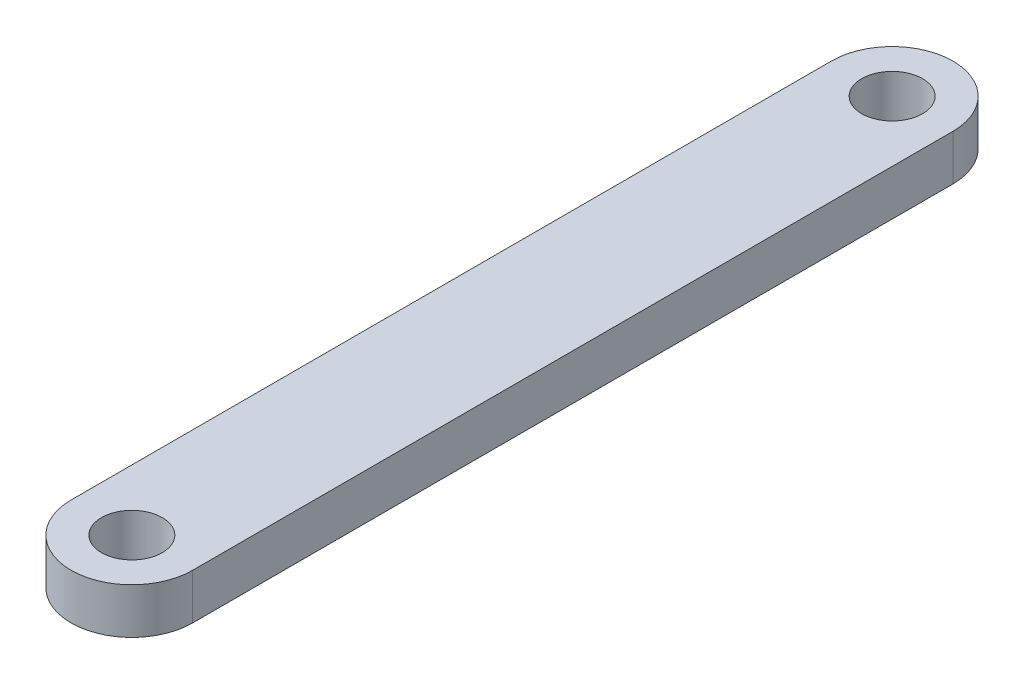
from build123d import *

# Parameters (mm, degrees)
SKETCH1_R           = 10
BOSS_EXTRUDE1_DEPTH = 15


with BuildPart() as part:
    # Sketch1 → Boss-Extrude1 (new body)
    with BuildSketch(Plane(origin=(0, 0, 0), x_dir=(1, 0, 0), z_dir=(0, 1, 0))):
        with BuildLine():
            Line((-20, 0), (-20, 250))
            ThreePointArc((-20, 250), (0, 270), (20, 250))
            Line((20, 250), (20, 0))
            ThreePointArc((20, 0), (0, -20), (-20, 0))
        make_face()
        with Locations(Location((0, 250, 0), (0, 0, 270))):
            Circle(SKETCH1_R, mode=Mode.SUBTRACT)
        with Locations(Location((0, 0, 0), (0, 0, 270))):
            Circle(SKETCH1_R, mode=Mode.SUBTRACT)
    extrude(amount=BOSS_EXTRUDE1_DEPTH)


solid = part.part
